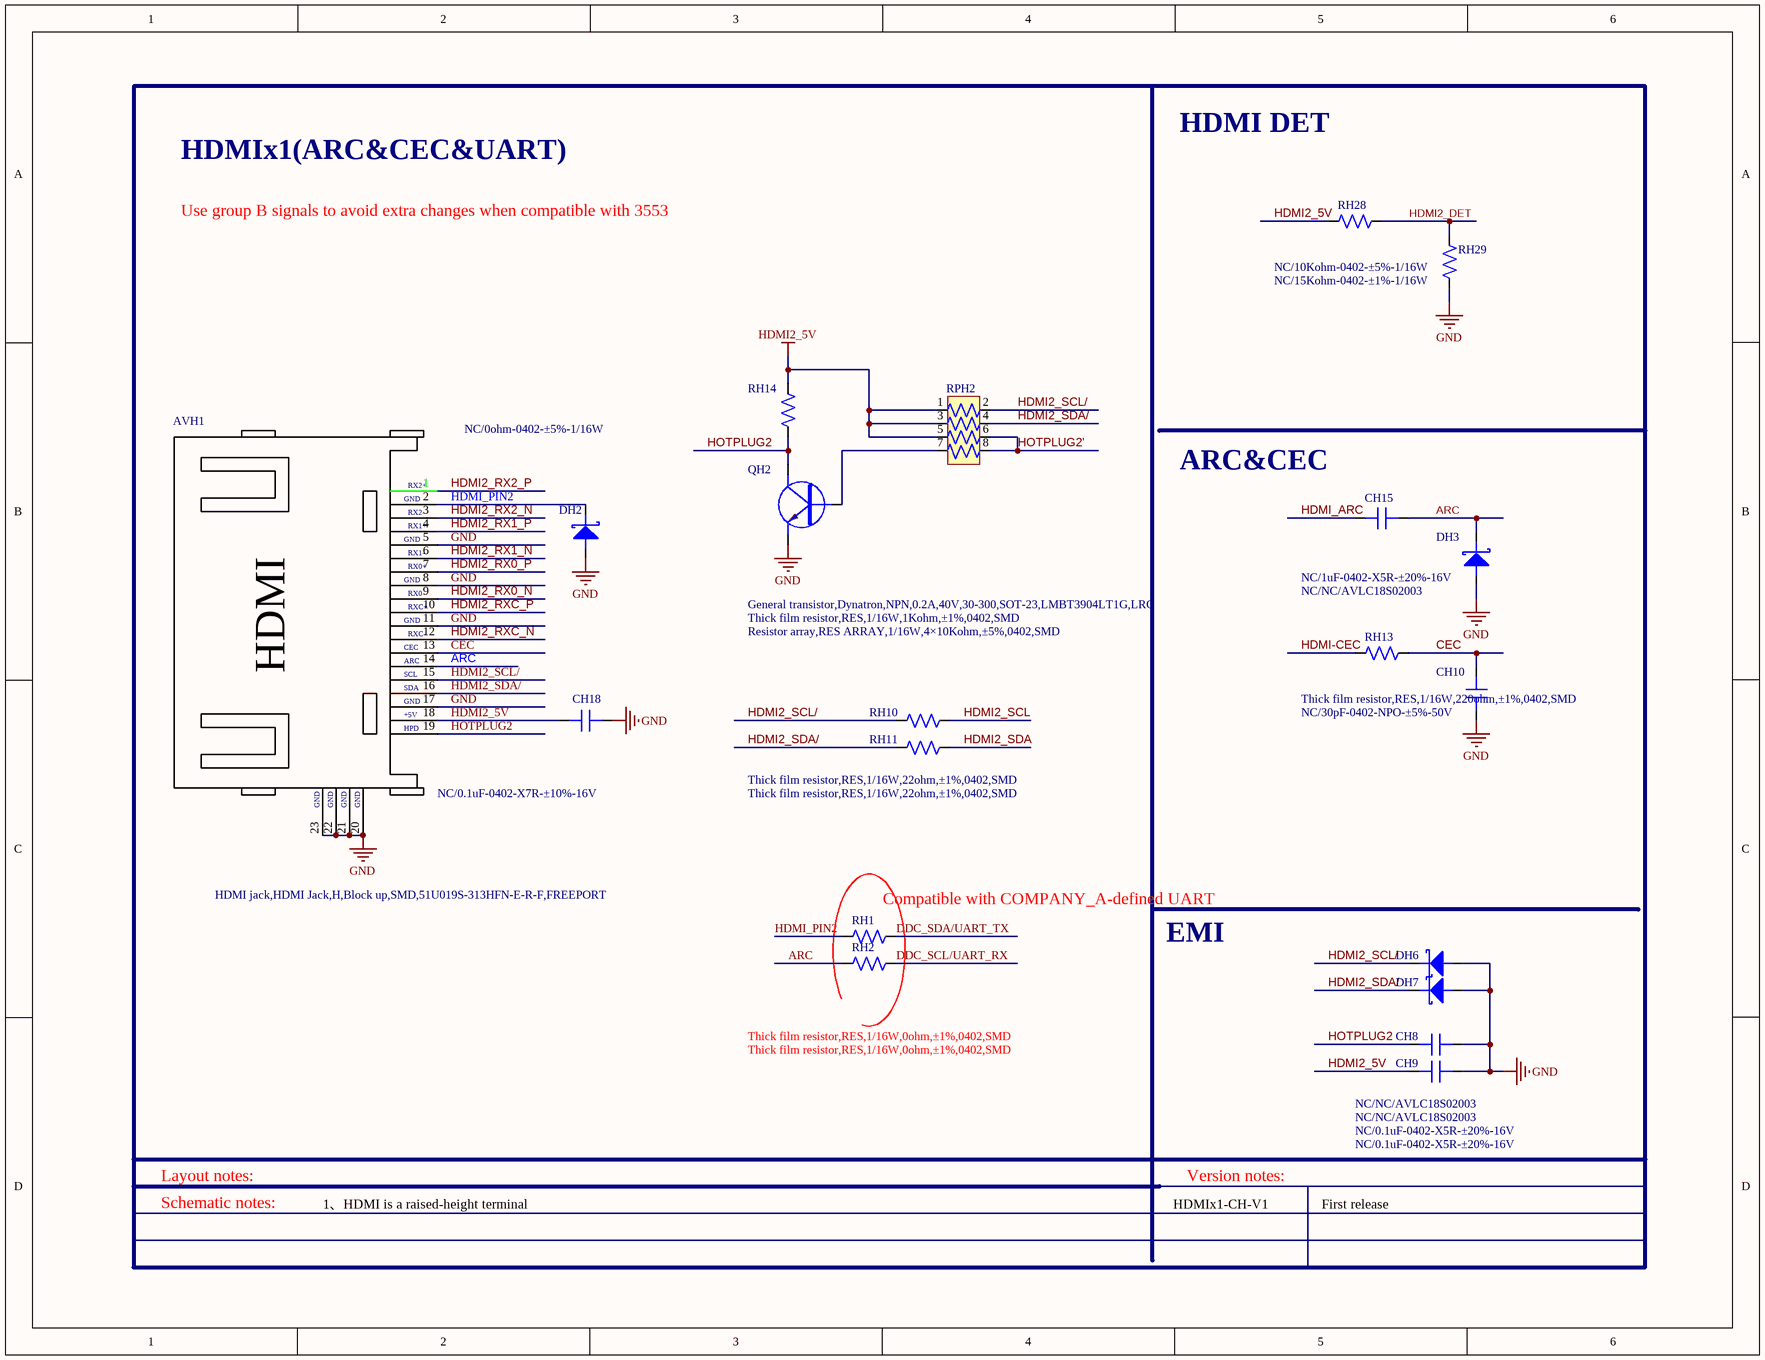
[diagram p0: MISC86383-14.SchDoc]
# Altium project MISC86383-33.PrjPCB (part 4 of 8)

## Sheet MISC86383-14.SchDoc
size 330 x 254 mm

### Parts
AVH1  HDMI jack,HDMI Jack,H,Block up,SMD,51U019S-313HFN-E-R-F,FREEPORT  [HDMI-HS-11]
CH8  NC/0.1uF-0402-X5R-±20%-16V  [C0402]
CH9  NC/0.1uF-0402-X5R-±20%-16V  [C0402]
CH10  NC/30pF-0402-NPO-±5%-50V  [C0402]
CH15  NC/1uF-0402-X5R-±20%-16V  [C0402]
CH18  NC/0.1uF-0402-X7R-±10%-16V  [C0402]
DH2  NC/0ohm-0402-±5%-1/16W  [DIODE-S0402]
DH3  NC/NC/AVLC18S02003  [DIODE-S0402]
DH6  NC/NC/AVLC18S02003  [DIODE-S0402]
DH7  NC/NC/AVLC18S02003  [DIODE-S0402]
QH2  General transistor,Dynatron,NPN,0.2A,40V,30-300,SOT-23,LMBT3904LT1G,LRC  [SOT-23]
RH1  Thick film resistor,RES,1/16W,0ohm,±1%,0402,SMD  [R0402]
RH2  Thick film resistor,RES,1/16W,0ohm,±1%,0402,SMD  [R0402]
RH10  Thick film resistor,RES,1/16W,22ohm,±1%,0402,SMD  [R0402]
RH11  Thick film resistor,RES,1/16W,22ohm,±1%,0402,SMD  [R0402]
RH13  Thick film resistor,RES,1/16W,220ohm,±1%,0402,SMD  [R0402]
RH14  Thick film resistor,RES,1/16W,1Kohm,±1%,0402,SMD  [R0402]
RH28  NC/10Kohm-0402-±5%-1/16W  [R0402]
RH29  NC/15Kohm-0402-±1%-1/16W  [R0402]
RPH2  Resistor array,RES ARRAY,1/16W,4×10Kohm,±5%,0402,SMD  [RA0402]

### Nets
GND: AVH1.5 AVH1.8 AVH1.11 AVH1.17 AVH1.20 AVH1.21 AVH1.22 AVH1.23 CH8.1 CH9.1 CH10.1 CH18.1 DH2.A DH3.A DH6.A DH7.A QH2.E RH29.2
HDMI2_5V: AVH1.18 CH9.2 CH18.2 RH14.2 RH28.2 RPH2.1 RPH2.3 RPH2.5
ARC: AVH1.14 CH15.1 DH3.K RH2.1
CEC: AVH1.13 CH10.2 RH13.1
DDC_SCL/UART_RX: RH2.2
DDC_SDA/UART_TX: RH1.2
HDMI2_DET: RH28.1 RH29.1
HDMI2_RX0_N: AVH1.9
HDMI2_RX0_P: AVH1.7
HDMI2_RX1_N: AVH1.6
HDMI2_RX1_P: AVH1.4
HDMI2_RX2_N: AVH1.3
HDMI2_RX2_P: AVH1.1
HDMI2_RXC_N: AVH1.12
HDMI2_RXC_P: AVH1.10
HDMI2_SCL: RH10.1
HDMI2_SCL/: AVH1.15 DH6.K RH10.2 RPH2.2
HDMI2_SDA: RH11.1
HDMI2_SDA/: AVH1.16 DH7.K RH11.2 RPH2.4
HDMI-CEC: RH13.2
HDMI_ARC: CH15.2
HDMI_PIN2: AVH1.2 DH2.K RH1.1
HOTPLUG2: AVH1.19 CH8.2 QH2.C RH14.1
HOTPLUG2': RPH2.6 RPH2.8
NetQH2_B: QH2.B RPH2.7

### Notes on the sheet
- HDMIx1(ARC&CEC&UART)
- HDMI DET
- Use group B signals to avoid extra changes when compatible with 3553
- ARC&CEC
- (near RH1) Compatible with COMPANY_A-defined UART
- EMI
- Layout notes:
- Schematic notes:
- 1、HDMI is a raised-height terminal
- HDMIx1-CH-V1
- Version notes:
- First release

### Library data of the parts
AVH1 = XXX.XXX.0001809-D: HDMI jack,HDMI Jack,H,Block up,SMD,51U019S-313HFN-E-R-F,FREEPORT-D
CH8 CH9 CH18 = 0.1uF-0402-Y5V-+80%-20%-16V-D
CH10 = 33pF-0402-NPO-±5%-50V-D
CH15 = 1uF-0402-X5R-±20%-16V-D
DH2 DH3 DH6 DH7 = AVLC18S02003-D
QH2 = MMBT3904(f≥350MHz)-D-NPN: Q-NPN-#-#-#
RH1 RH2 = 0ohm-0402-±5%-1/16W-D
RH10 RH11 = 10Kohm-0402-±5%-1/16W-D
RH13 RH28 RH29 = 220ohm-0402-±5%-1/16W-D
RH14 = 1Kohm-0402-±5%-1/16W-D
RPH2 = 4*100ohm-0402-±5%-1/16W-D

## Sheet MISC86383-15.SchDoc
size 330 x 228 mm
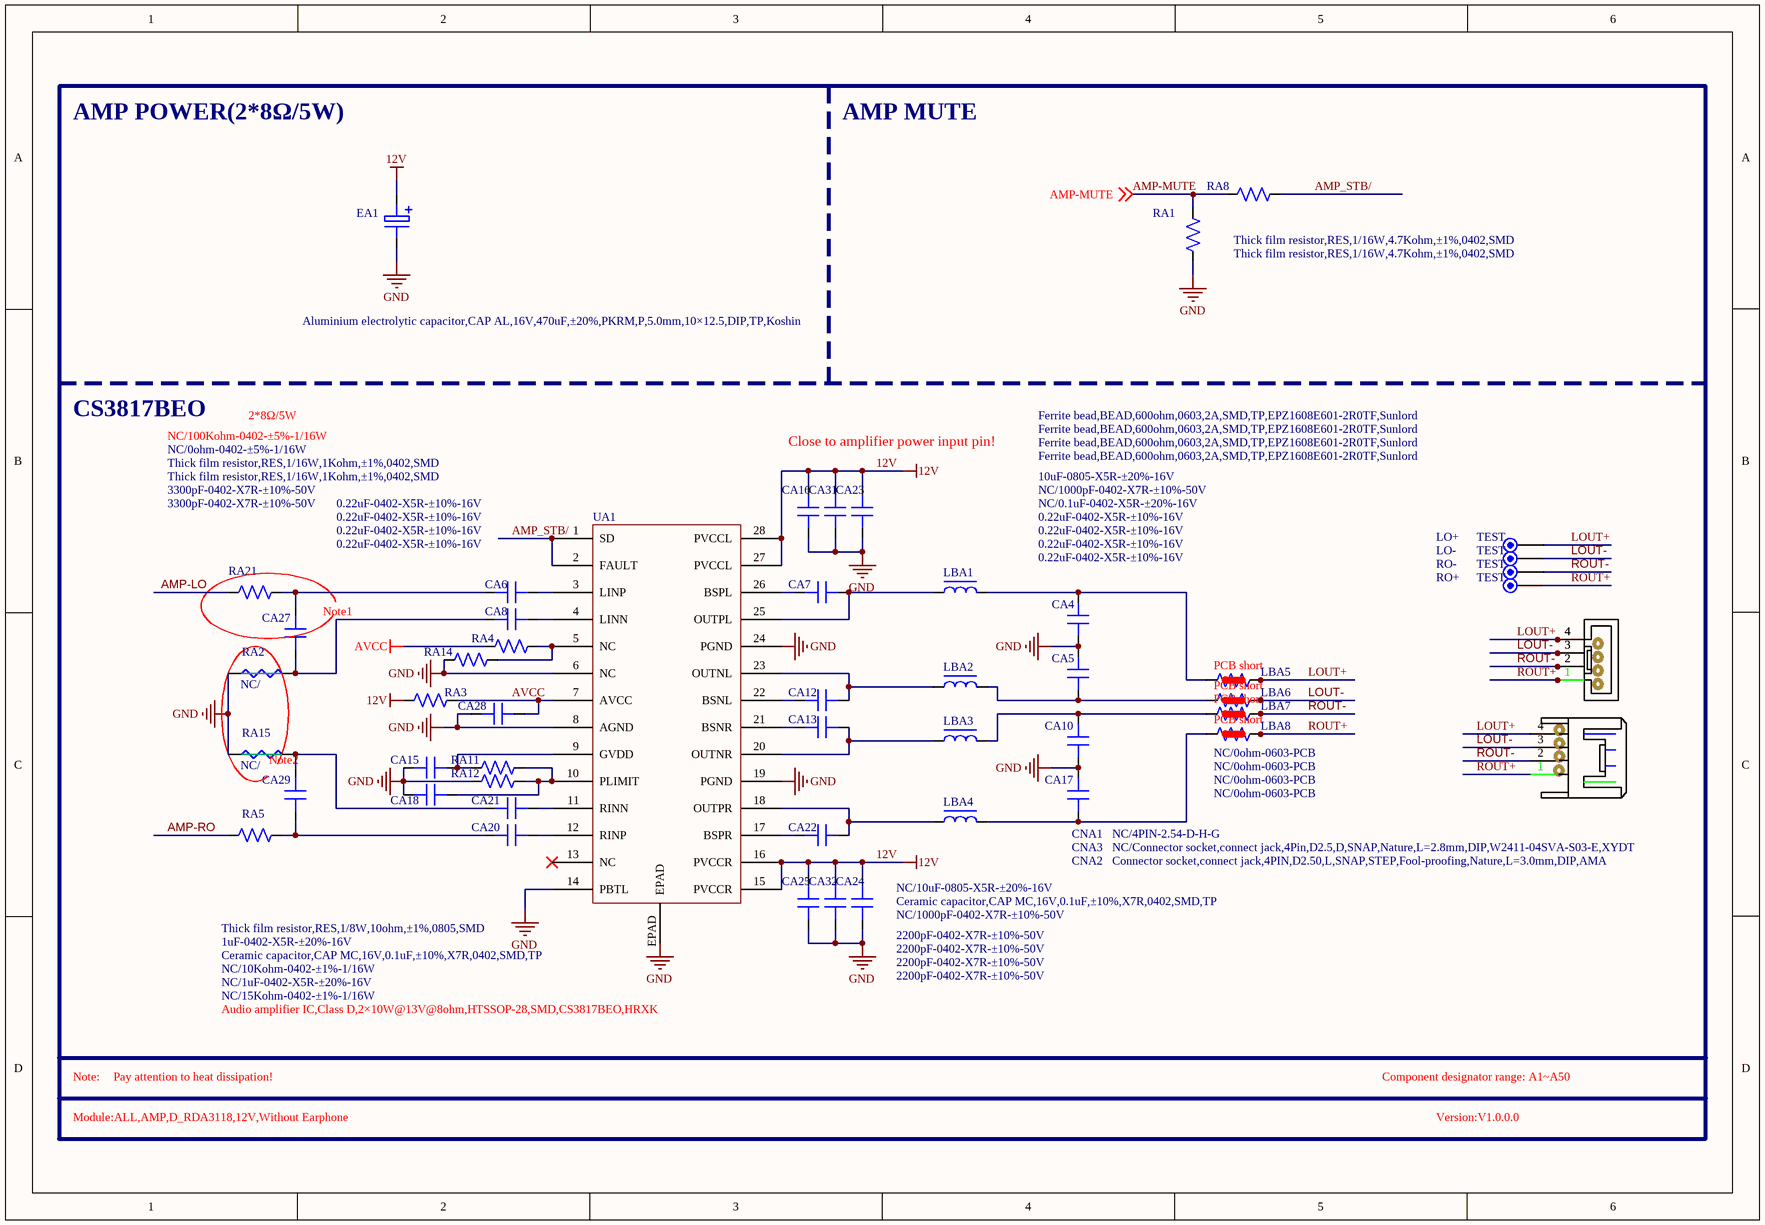
[diagram p1: MISC86383-15.SchDoc]

### Parts
CA4  2200pF-0402-X7R-±10%-50V  [C0402]
CA5  2200pF-0402-X7R-±10%-50V  [C0402]
CA6  0.22uF-0402-X5R-±10%-16V  [C0402]
CA7  0.22uF-0402-X5R-±10%-16V  [C0402]
CA8  0.22uF-0402-X5R-±10%-16V  [C0402]
CA10  2200pF-0402-X7R-±10%-50V  [C0402]
CA12  0.22uF-0402-X5R-±10%-16V  [C0402]
CA13  0.22uF-0402-X5R-±10%-16V  [C0402]
CA15  Ceramic capacitor,CAP MC,16V,0.1uF,±10%,X7R,0402,SMD,TP  [C0402]
CA16  NC/1000pF-0402-X7R-±10%-50V  [C0402]
CA17  2200pF-0402-X7R-±10%-50V  [C0402]
CA18  NC/1uF-0402-X5R-±20%-16V  [C0402]
CA20  0.22uF-0402-X5R-±10%-16V  [C0402]
CA21  0.22uF-0402-X5R-±10%-16V  [C0402]
CA22  0.22uF-0402-X5R-±10%-16V  [C0402]
CA23  NC/0.1uF-0402-X5R-±20%-16V  [C0402]
CA24  Ceramic capacitor,CAP MC,16V,0.1uF,±10%,X7R,0402,SMD,TP  [C0402]
CA25  NC/1000pF-0402-X7R-±10%-50V  [C0402]
CA27  3300pF-0402-X7R-±10%-50V  [C0402]
CA28  1uF-0402-X5R-±20%-16V  [C0402]
CA29  3300pF-0402-X7R-±10%-50V  [C0402]
CA31  10uF-0805-X5R-±20%-16V  [C0805]
CA32  NC/10uF-0805-X5R-±20%-16V  [C0805]
CNA1  NC/4PIN-2.54-D-H-G  [SIP4/2.54D-1]
CNA2  Connector socket,connect jack,4PIN,D2.50,L,SNAP,STEP,Fool-proofing,Nature,L=3.0mm,DIP,AMA  [SIP4H/2.5D-7]
CNA3  NC/Connector socket,connect jack,4Pin,D2.5,D,SNAP,Nature,L=2.8mm,DIP,W2411-04SVA-S03-E,XYDT  [SIP4/2.5D-2]
EA1  Aluminium electrolytic capacitor,CAP AL,16V,470uF,±20%,PKRM,P,5.0mm,10×12.5,DIP,TP,Koshin  [EC(10*12.5)-V-5]
LBA1  Ferrite bead,BEAD,600ohm,0603,2A,SMD,TP,EPZ1608E601-2R0TF,Sunlord  [L0603]
LBA2  Ferrite bead,BEAD,600ohm,0603,2A,SMD,TP,EPZ1608E601-2R0TF,Sunlord  [L0603]
LBA3  Ferrite bead,BEAD,600ohm,0603,2A,SMD,TP,EPZ1608E601-2R0TF,Sunlord  [L0603]
LBA4  Ferrite bead,BEAD,600ohm,0603,2A,SMD,TP,EPZ1608E601-2R0TF,Sunlord  [L0603]
LBA5  NC/0ohm-0603-PCB  [R0603SC]
LBA6  NC/0ohm-0603-PCB  [R0603SC]
LBA7  NC/0ohm-0603-PCB  [R0603SC]
LBA8  NC/0ohm-0603-PCB  [R0603SC]
LO+  TEST  [TP]
LO-  TEST  [TP]
RA1  Thick film resistor,RES,1/16W,4.7Kohm,±1%,0402,SMD  [R0402]
RA2  NC/  [GND]
RA3  Thick film resistor,RES,1/8W,10ohm,±1%,0805,SMD  [R0805]
RA4  NC/100Kohm-0402-±5%-1/16W  [R0402]
RA5  Thick film resistor,RES,1/16W,1Kohm,±1%,0402,SMD  [R0402]
RA8  Thick film resistor,RES,1/16W,4.7Kohm,±1%,0402,SMD  [R0402]
RA11  NC/10Kohm-0402-±1%-1/16W  [R0402]
RA12  NC/15Kohm-0402-±1%-1/16W  [R0402]
RA14  NC/0ohm-0402-±5%-1/16W  [R0402]
RA15  NC/  [GND]
RA21  Thick film resistor,RES,1/16W,1Kohm,±1%,0402,SMD  [R0402]
RO+  TEST  [TP]
RO-  TEST  [TP]
UA1  Audio amplifier IC,Class D,2×10W@13V@8ohm,HTSSOP-28,SMD,CS3817BEO,HRXK  [SSOP28/0.65-5]

### Nets
12V: CA16.2 CA23.2 CA24.2 CA25.2 CA31.2 CA32.2 EA1.1 RA3.1 UA1.15(PVCCR) UA1.16(PVCCR) UA1.27(PVCCL) UA1.28(PVCCL)
AVCC: CA28.2 RA3.2 RA4.2 UA1.7(AVCC)
GND: CA4.2 CA5.2 CA10.2 CA15.2 CA16.1 CA17.1 CA18.2 CA23.1 CA24.1 CA25.1 CA28.1 CA31.1 CA32.1 EA1.2 RA1.1 RA2.JP_2K RA12.2 RA14.1 RA15.JP_2K UA1.6(NC) UA1.8(AGND) UA1.14(PBTL) UA1.19(PGND) UA1.24(PGND) UA1.EPAD
AMP-LO: RA21.1
AMP-MUTE: RA1.2 RA8.1 ; off-sheet AMP-MUTE
AMP-RO: RA5.1
AMP_STB/: RA8.2 UA1.1(SD) UA1.2(FAULT)
LOUT+: CNA1.4 CNA2.4 CNA3.4 LBA5.2 LBA5.3 LO+.1
LOUT-: CNA1.3 CNA2.3 CNA3.3 LBA6.2 LBA6.3 LO-.1
ROUT+: CNA1.1 CNA2.1 CNA3.1 LBA8.2 LBA8.3 RO+.1
ROUT-: CNA1.2 CNA2.2 CNA3.2 LBA7.2 LBA7.3 RO-.1
NetCA4_1: CA4.1 LBA1.2 LBA5.1
NetCA5_1: CA5.1 LBA2.2 LBA6.1
NetCA6_1: CA6.1 UA1.3(LINP)
NetCA6_2: CA6.2 CA27.1 RA21.2
NetCA7_1: CA7.1 UA1.26(BSPL)
NetCA7_2: CA7.2 LBA1.1 UA1.25(OUTPL)
NetCA8_1: CA8.1 UA1.4(LINN)
NetCA8_2: CA8.2 CA27.2 RA2.JP_1K
NetCA10_1: CA10.1 LBA3.2 LBA7.1
NetCA12_1: CA12.1 UA1.22(BSNL)
NetCA12_2: CA12.2 LBA2.1 UA1.23(OUTNL)
NetCA13_1: CA13.1 UA1.21(BSNR)
NetCA13_2: CA13.2 LBA3.1 UA1.20(OUTNR)
NetCA15_1: CA15.1 RA11.2 UA1.9(GVDD)
NetCA17_2: CA17.2 LBA4.2 LBA8.1
NetCA18_1: CA18.1 RA11.1 RA12.1 UA1.10(PLIMIT)
NetCA20_1: CA20.1 UA1.12(RINP)
NetCA20_2: CA20.2 CA29.1 RA5.2
NetCA21_1: CA21.1 UA1.11(RINN)
NetCA21_2: CA21.2 CA29.2 RA15.JP_1K
NetCA22_1: CA22.1 UA1.17(BSPR)
NetCA22_2: CA22.2 LBA4.1 UA1.18(OUTPR)
NetRA4_1: RA4.1 RA14.2 UA1.5(NC)

Not connected (* = marked no-connect by the designer): UA1 13(NC)*

### Notes on the sheet
- AMP POWER(2*8Ω/5W)
- AMP MUTE
- CS3817BEO
- 2*8Ω/5W
- Close to amplifier power input pin!
- (near CA27) Note1
- (near RA15) Note2
- Note:
- Pay attention to heat dissipation!
- Component designator range: A1~A50
- Module:ALL,AMP,D_RDA3118,12V,Without Earphone
- Version:V1.0.0.0

### Library data of the parts
CA4 CA5 CA10 CA16 CA17 CA25 CA27 CA29 = 1000pF-0402-X7R-±10%-50V-D
CA6 CA8 CA20 CA21 = 0.22uF-0402-X5R-±10%-16V-D
CA7 CA12 CA13 CA22 = 0.22uF-0402-Y5V-+80%-20%-16V-D
CA15 CA18 = 1uF-0402-X5R-±20%-16V-D
CA23 CA24 CA28 = 0.1uF-0402-Y5V-+80%-20%-16V-D
CA31 CA32 = 10uF-0603-X5R-±20%-6.3V-D
CNA1 = 4PIN-2.54-D-H-G-DHMI
CNA2 = XXX.XXX.0001836-DLMI: Connector socket,connect jack,4PIN,D2.50,L,SNAP,STEP,Fool-proofing,Nature,L=3.0mm,DIP,AMA-DLMI
CNA3 = 4PIN-2.54-D-H-G-带扣-B-DHMI
EA1 = 470uF-25V-±20%-10×12-105℃-YE-编带-F=5.0(Elite)-DHAI: Electrolytic
LBA1-LBA4 = 004.004.0000104-D: Multilayer inductor,HF Inductor,220nH,±5%,0603,SMD,SWI0603F-R22J,Tai-tech-D
LBA5-LBA8 = 0ohm-0603-PCB-D
RA1 RA8 = 100ohm-0402-±5%-1/16W-D
RA2 RA15 = GND: Manufacturer: Panasonic; Part Number: ERJ3GEYJ473V; Right: 20; Bottom: 30; CLASS: Discrete; Comments: Digikey
RA3 = 10ohm-0805-±5%-1/8W-D
RA4 = 47Kohm-0402-±5%-1/16W-D
RA5 RA21 = 180ohm-0402-±5%-1/16W-D
RA11 = 12Kohm-0402-±5%-1/16W-D
RA12 = 9K1ohm-0402-±5%-1/16W-D
RA14 = 0ohm-0402-±5%-1/16W-D
UA1 = 音频功放,IC Audio AMP,Class D,2×9W@13V@8ohm,HTSSOP28,SMD,TPA3136D2,TI-D

## Sheet MISC86383-16.SchDoc
size 482 x 304 mm
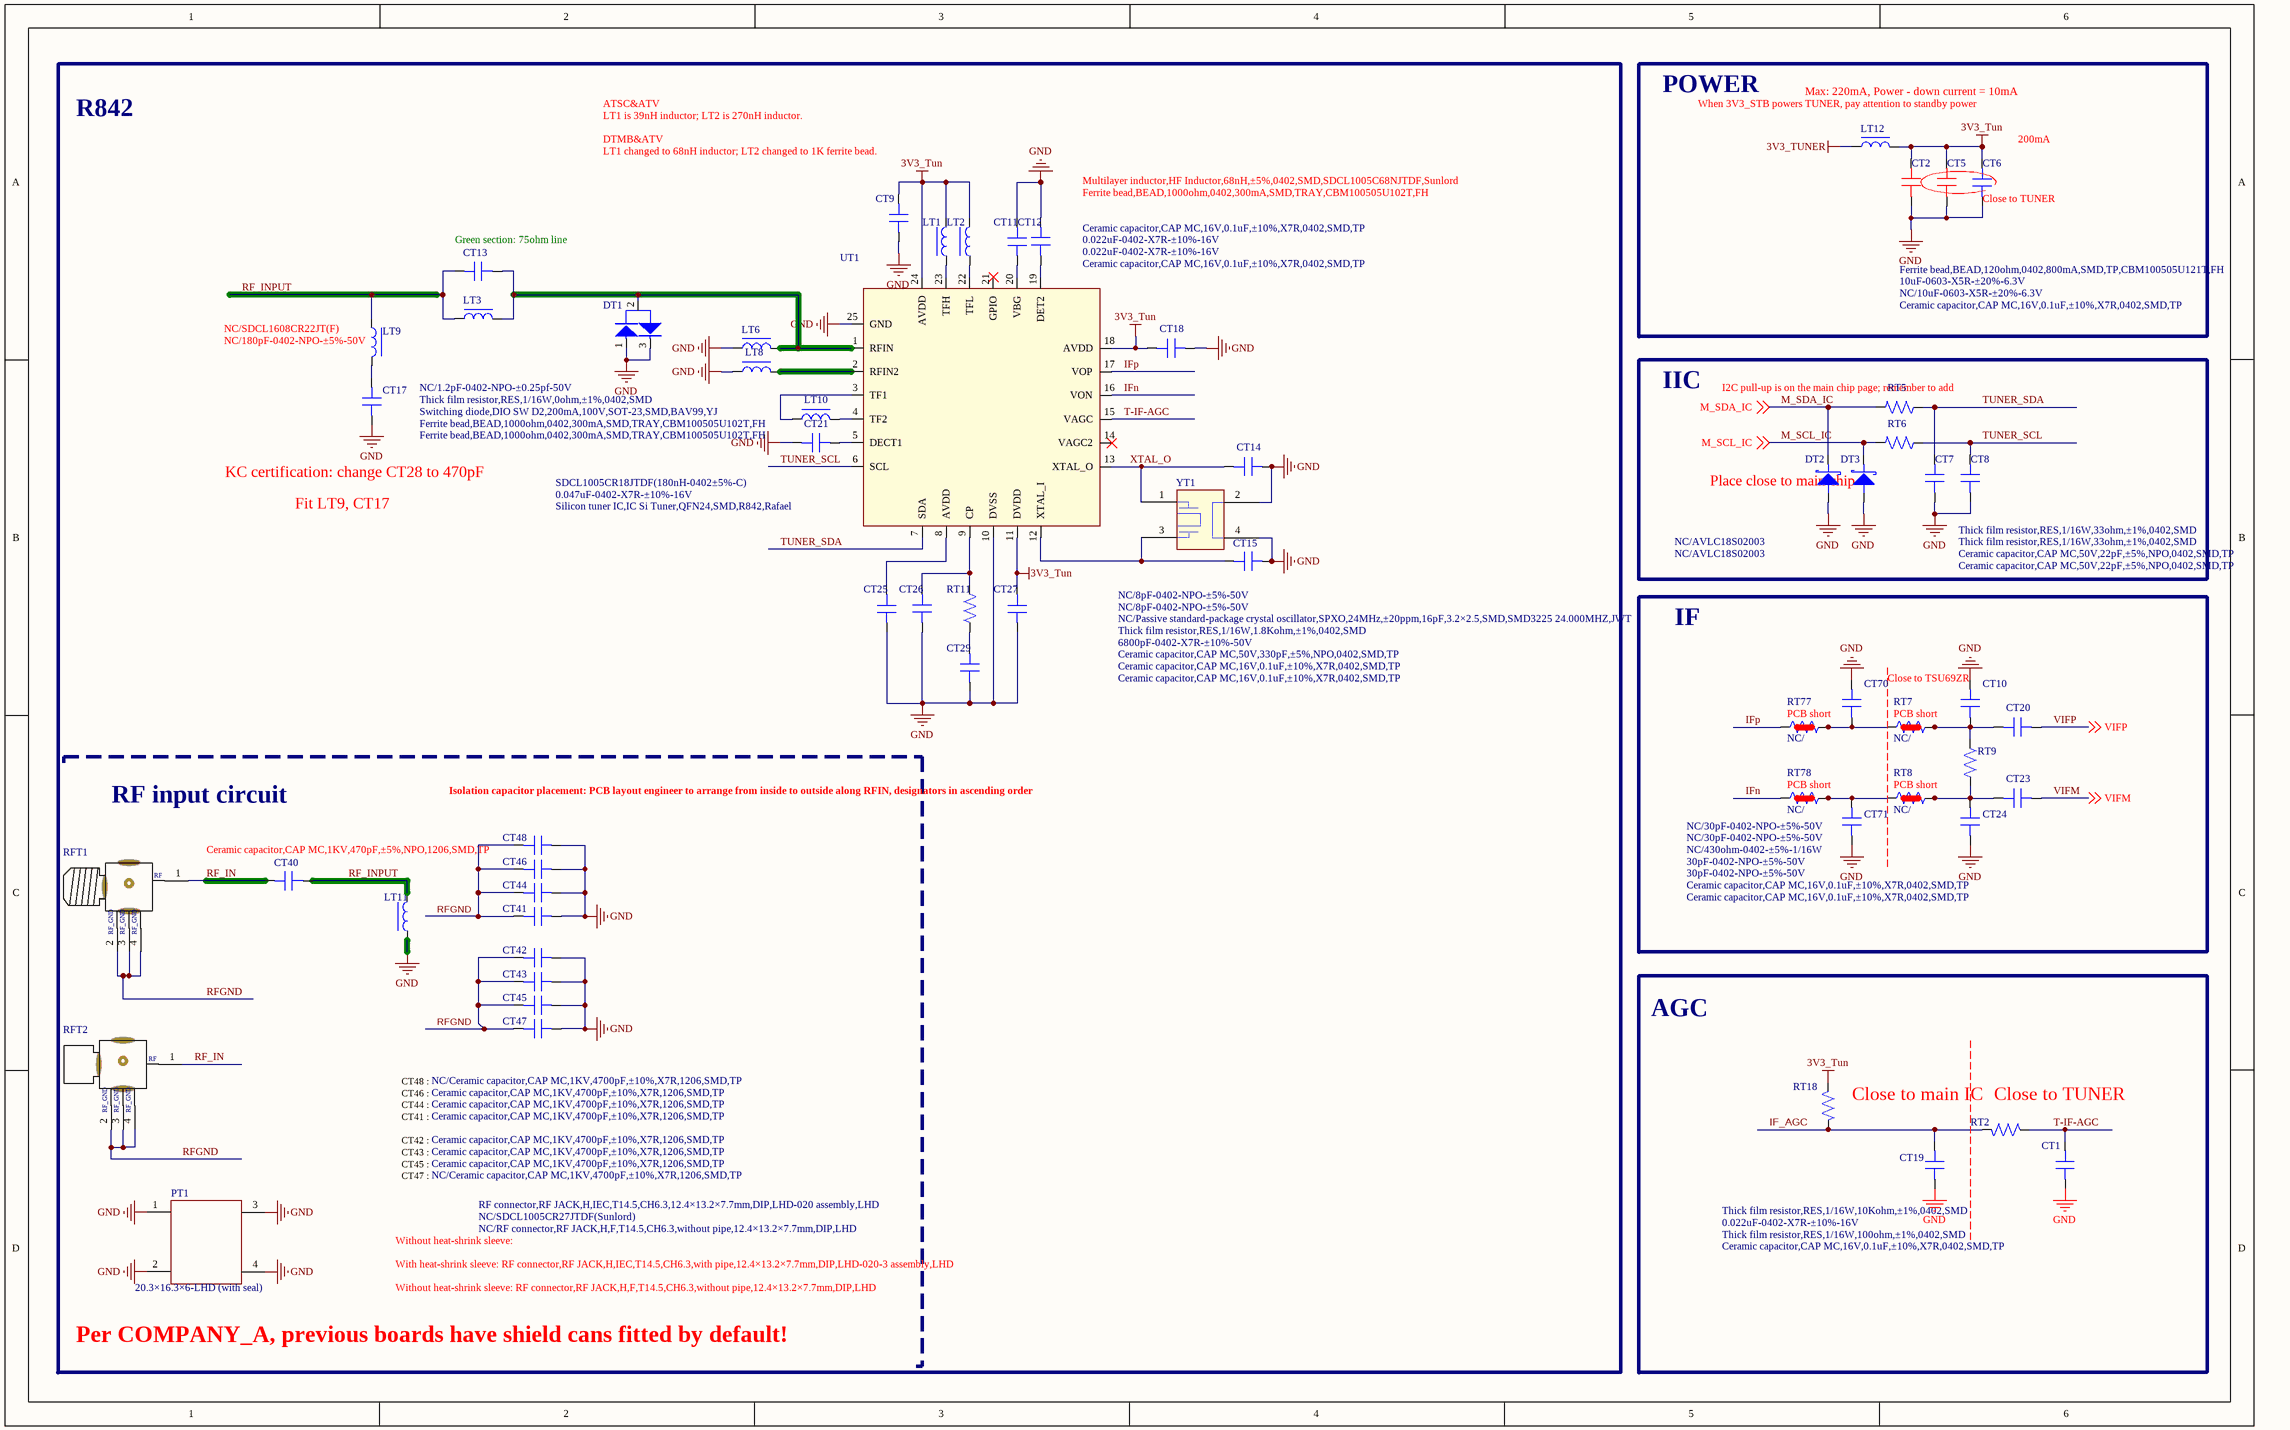
[diagram p2: MISC86383-16.SchDoc]

### Parts
CT1  Ceramic capacitor,CAP MC,16V,0.1uF,±10%,X7R,0402,SMD,TP  [C0402]
CT2  10uF-0603-X5R-±20%-6.3V  [C0603]
CT5  NC/10uF-0603-X5R-±20%-6.3V  [C0603]
CT6  Ceramic capacitor,CAP MC,16V,0.1uF,±10%,X7R,0402,SMD,TP  [C0402]
CT7  Ceramic capacitor,CAP MC,50V,22pF,±5%,NPO,0402,SMD,TP  [C0402]
CT8  Ceramic capacitor,CAP MC,50V,22pF,±5%,NPO,0402,SMD,TP  [C0402]
CT9  Ceramic capacitor,CAP MC,16V,0.1uF,±10%,X7R,0402,SMD,TP  [C0402]
CT10  30pF-0402-NPO-±5%-50V  [C0402]
CT11  0.022uF-0402-X7R-±10%-16V  [C0402]
CT12  0.022uF-0402-X7R-±10%-16V  [C0402]
CT13  NC/1.2pF-0402-NPO-±0.25pf-50V  [C0402]
CT14  NC/8pF-0402-NPO-±5%-50V  [C0402]
CT15  NC/8pF-0402-NPO-±5%-50V  [C0402]
CT17  NC/180pF-0402-NPO-±5%-50V  [C0402]
CT18  Ceramic capacitor,CAP MC,16V,0.1uF,±10%,X7R,0402,SMD,TP  [C0402]
CT19  0.022uF-0402-X7R-±10%-16V  [C0402]
CT20  Ceramic capacitor,CAP MC,16V,0.1uF,±10%,X7R,0402,SMD,TP  [C0402]
CT21  0.047uF-0402-X7R-±10%-16V  [C0402]
CT23  Ceramic capacitor,CAP MC,16V,0.1uF,±10%,X7R,0402,SMD,TP  [C0402]
CT24  30pF-0402-NPO-±5%-50V  [C0402]
CT25  Ceramic capacitor,CAP MC,16V,0.1uF,±10%,X7R,0402,SMD,TP  [C0402]
CT26  Ceramic capacitor,CAP MC,50V,330pF,±5%,NPO,0402,SMD,TP  [C0402]
CT27  Ceramic capacitor,CAP MC,16V,0.1uF,±10%,X7R,0402,SMD,TP  [C0402]
CT29  6800pF-0402-X7R-±10%-50V  [C0402]
CT40  Ceramic capacitor,CAP MC,1KV,470pF,±5%,NPO,1206,SMD,TP  [C1206]
CT41  Ceramic capacitor,CAP MC,1KV,4700pF,±10%,X7R,1206,SMD,TP  [C1206]
CT42  Ceramic capacitor,CAP MC,1KV,4700pF,±10%,X7R,1206,SMD,TP  [C1206]
CT43  Ceramic capacitor,CAP MC,1KV,4700pF,±10%,X7R,1206,SMD,TP  [C1206]
CT44  Ceramic capacitor,CAP MC,1KV,4700pF,±10%,X7R,1206,SMD,TP  [C1206]
CT45  Ceramic capacitor,CAP MC,1KV,4700pF,±10%,X7R,1206,SMD,TP  [C1206]
CT46  Ceramic capacitor,CAP MC,1KV,4700pF,±10%,X7R,1206,SMD,TP  [C1206]
CT47  NC/Ceramic capacitor,CAP MC,1KV,4700pF,±10%,X7R,1206,SMD,TP  [C1206]
CT48  NC/Ceramic capacitor,CAP MC,1KV,4700pF,±10%,X7R,1206,SMD,TP  [C1206]
CT70  NC/30pF-0402-NPO-±5%-50V  [C0402]
CT71  NC/30pF-0402-NPO-±5%-50V  [C0402]
DT1  Switching diode,DIO SW D2,200mA,100V,SOT-23,SMD,BAV99,YJ  [SO-23]
DT2  NC/AVLC18S02003  [DIODE-S0402]
DT3  NC/AVLC18S02003  [DIODE-S0402]
LT1  Multilayer inductor,HF Inductor,68nH,±5%,0402,SMD,SDCL1005C68NJTDF,Sunlord  [L0402]
LT2  Ferrite bead,BEAD,1000ohm,0402,300mA,SMD,TRAY,CBM100505U102T,FH  [L0402]
LT3  Thick film resistor,RES,1/16W,0ohm,±1%,0402,SMD  [L0402]
LT6  Ferrite bead,BEAD,1000ohm,0402,300mA,SMD,TRAY,CBM100505U102T,FH  [L0402]
LT8  Ferrite bead,BEAD,1000ohm,0402,300mA,SMD,TRAY,CBM100505U102T,FH  [L0402]
LT9  NC/SDCL1608CR22JT(F)  [L0603]
LT10  SDCL1005CR18JTDF(180nH-0402±5%-C)  [L0402]
LT11  NC/SDCL1005CR27JTDF(Sunlord)  [L0402]
LT12  Ferrite bead,BEAD,120ohm,0402,800mA,SMD,TP,CBM100505U121T,FH  [L0402]
PT1  20.3×16.3×6-LHD (with seal)  [SHIELD(16*20*6)]
RFT1  NC/RF connector,RF JACK,H,F,T14.5,CH6.3,without pipe,12.4×13.2×7.7mm,DIP,LHD  [T-13.2×12.4×7.7-F14.5]
RFT2  RF connector,RF JACK,H,IEC,T14.5,CH6.3,12.4×13.2×7.7mm,DIP,LHD-020 assembly,LHD  [ANT-IEC14.5-H-4]
RT2  Thick film resistor,RES,1/16W,100ohm,±1%,0402,SMD  [R0402]
RT5  Thick film resistor,RES,1/16W,33ohm,±1%,0402,SMD  [R0402]
RT6  Thick film resistor,RES,1/16W,33ohm,±1%,0402,SMD  [R0402]
RT7  NC/  [R0402SC]
RT8  NC/  [R0402SC]
RT9  NC/430ohm-0402-±5%-1/16W  [R0402]
RT11  Thick film resistor,RES,1/16W,1.8Kohm,±1%,0402,SMD  [R0402]
RT18  Thick film resistor,RES,1/16W,10Kohm,±1%,0402,SMD  [R0402]
RT77  NC/  [R0402SC]
RT78  NC/  [R0402SC]
UT1  Silicon tuner IC,IC Si Tuner,QFN24,SMD,R842,Rafael  [QFN24/0.5-3]
YT1  NC/Passive standard-package crystal oscillator,SPXO,24MHz,±20ppm,16pF,3.2×2.5,SMD,SMD3225 24.000MHZ,JWT  [XTAL-S-10]

### Blocks framed on the sheet
POWER: CT2 CT5 CT6 LT12
IIC: CT7 CT8 DT2 DT3 RT5 RT6
IF: CT10 CT20 CT23 CT24 CT70 CT71 RT7-RT9 RT77 RT78
AGC: CT1 CT19 RT2 RT18

### Nets
3V3_Tun: CT2.2 CT5.2 CT6.1 CT9.1 CT18.2 CT27.1 LT1.1 LT2.2 LT12.2 RT18.1 UT1.11(DVDD) UT1.18(AVDD) UT1.24(AVDD)
3V3_TUNER: LT12.1
GND: CT1.1 CT2.1 CT5.1 CT6.2 CT7.1 CT8.1 CT9.2 CT10.2 CT11.1 CT12.2 CT14.1 CT15.1 CT17.2 CT18.1 CT19.1 CT21.2 CT24.1 CT25.2 CT26.1 CT27.2 CT29.1 CT41.1 CT42.1 CT43.1 CT44.1 CT45.1 CT46.1 CT47.1 CT48.1 CT70.2 CT71.1 DT1.1 DT1.3 DT2.A DT3.A LT6.2 LT8.2 LT11.2 PT1.1 PT1.2 PT1.3 PT1.4 UT1.10(DVSS) UT1.25(GND) YT1.2 YT1.4
IF_AGC: CT19.2 RT2.2 RT18.2
IFn: RT78.1 UT1.16(VON)
IFp: RT77.1 UT1.17(VOP)
M_SCL_IC: DT3.K RT6.2 ; off-sheet M_SCL_IC
M_SDA_IC: DT2.K RT5.2 ; off-sheet M_SDA_IC
RF_IN: CT40.1 RFT1.1 RFT2.1
RF_INPUT: CT13.1 CT40.2 LT3.1 LT9.1 LT11.1
RFGND: CT41.2 CT42.2 CT43.2 CT44.2 CT45.2 CT46.2 CT47.2 CT48.2 RFT1.2 RFT1.3 RFT1.4 RFT2.2 RFT2.3 RFT2.4
T-IF-AGC: CT1.2 RT2.1 UT1.15(VAGC)
TUNER_SCL: CT8.2 RT6.1 UT1.6(SCL)
TUNER_SDA: CT7.2 RT5.1 UT1.7(SDA)
VIFM: CT23.2 ; off-sheet VIFM
VIFP: CT20.2 ; off-sheet VIFP
XTAL_O: CT14.2 UT1.13(XTAL_O) YT1.1
NetCT10_1: CT10.1 CT20.1 RT7.2 RT7.3 RT9.1
NetCT11_2: CT11.2 UT1.20(VBG)
NetCT12_1: CT12.1 UT1.19(DET2)
NetCT13_2: CT13.2 DT1.2 LT3.2 LT6.1 UT1.1(RFIN)
NetCT15_2: CT15.2 UT1.12(XTAL_I) YT1.3
NetCT17_1: CT17.1 LT9.2
NetCT21_1: CT21.1 UT1.5(DECT1)
NetCT23_1: CT23.1 CT24.2 RT8.2 RT8.3 RT9.2
NetCT25_1: CT25.1 UT1.8(AVDD)
NetCT26_2: CT26.2 RT11.2 UT1.9(CP)
NetCT29_2: CT29.2 RT11.1
NetCT70_1: CT70.1 RT7.1 RT77.2 RT77.3
NetCT71_2: CT71.2 RT8.1 RT78.2 RT78.3
NetLT1_2: LT1.2 UT1.23(TFH)
NetLT2_1: LT2.1 UT1.22(TFL)
NetLT8_1: LT8.1 UT1.2(RFIN2)
NetLT10_1: LT10.1 UT1.4(TF2)
NetLT10_2: LT10.2 UT1.3(TF1)

Not connected (* = marked no-connect by the designer): UT1 14(VAGC2)* 21(GPIO)*

### Notes on the sheet
- R842
- ATSC&ATV
- DTMB&ATV
- LT1 is 39nH inductor; LT2 is 270nH inductor.
- When 3V3_STB powers TUNER, pay attention to standby power
- Max: 220mA, Power - down current = 10mA
- (near CT6) 200mA
- (near CT9) LT1 changed to 68nH inductor; LT2 changed to 1K ferrite bead.
- (near CT6) Close to TUNER
- (near CT13) Green section: 75ohm line
- (near RT5) I2C pull-up is on the main chip page; remember to add
- KC certification: change CT28 to 470pF
- Place close to main chip
- Fit LT9, CT17
- (near CT10) Close to TSU69ZR
- Isolation capacitor placement: PCB layout engineer to arrange from inside to outside along RFIN, designators in ascending order
- RF input circuit
- CT46 :
- CT48 :
- CT41 :
- CT42 :
- CT44 :
- Close to main IC
- (near RT2) Close to TUNER
- CT43 :
- CT45 :
- CT47 :
- With heat-shrink sleeve: RF connector,RF JACK,H,IEC,T14.5,CH6.3,with pipe,12.4×13.2×7.7mm,DIP,LHD-020-3 assembly,LHD
- Without heat-shrink sleeve:
- Without heat-shrink sleeve: RF connector,RF JACK,H,F,T14.5,CH6.3,without pipe,12.4×13.2×7.7mm,DIP,LHD
- Per COMPANY_A, previous boards have shield cans fitted by default!

### Library data of the parts
CT1 CT9 CT11 CT18 CT20 CT21 CT23 CT25 CT27 = 0.1uF-0402-Y5V-+80%-20%-16V-D
CT2 CT5 = 004.003.0000383-D: Ceramic capacitor,CAP MC,6.3V,10uF,±20%,X5R,0603,SMD,TP-D
CT6 = 1uF-0402-X5R-±20%-6.3V-D
CT7 CT8 = 004.003.0000530-D: Ceramic capacitor,CAP MC,50V,22pF,±5%,NPO,0402,SMD,TP-D
CT10 CT24 CT70 CT71 = 56pF-0402-NPO-±5%-50V-D
CT12 CT19 = 0.022uF-0402-X7R-±10%-16V-D
CT13 = 1.8pF-0402-NPO-±0.25pF-50V-D
CT14 CT15 = 8pF-0402-NPO-±5%-50V-D
CT17 = 120pF-0402-NPO-±5%-50V-D
CT26 = 330pF-0402-NPO-±5%-50V-D
CT29 = 6800pF-0402-X7R-±10%-50V-D
CT40 = 4700pF-1206-X7R-±10%-1000V-D
CT41-CT48 = 1000pF-1206-X7R-±20%-2000V-D
DT1 = BAV99-BR-D
DT2 DT3 = AVLC18S02003-D
LT1 = SDCL1005C68NJTDF(68nH-0402±5%-C)-D
LT2 LT6 LT8 = 1Kohm-0402-±25%-D
LT3 = 2.2nH-0402-±0.3nH-1/4-D
LT9 = SDCL1005CR33JTDF-D
LT10 = SDCL1608CR22JT(F)-D
LT11 = SDCL1005CR27JTDF(顺络)-D
LT12 = GZ1005U121CTF(120ohm-500mA)-D
PT1 = 20.3×16.3×6-LHD(带封口)-DMI
RFT1 = RF头,RF JACK,H,F,T14.5,CH6.3,without pipe,12.4×13.2×7.7mm,DIP,LHD-DLMI: T-F-6.3mm-#-#
RFT2 = RF头,RF JACK,H,IEC,T14.5,CH6.3,12.4×13.2×7.7mm,DIP,LHD-020组件,LHD-DLMI: T-IEC-6.3mm-#-#
RT2 RT18 = 10Kohm-0402-±5%-1/16W-D
RT5 RT6 = 33ohm-0402-±5%-1/16W-D
RT7 RT8 RT77 RT78 = 0ohm-0402-PCB-D
RT9 = 220ohm-0402-±5%-1/16W-D
RT11 = 1K8ohm-0402-±5%-1/16W-D
UT1 = R840-D
YT1 = 004.009.0000056: Passive standard-package crystal oscillator,SPXO,24MHz,±20ppm,16pF,3.2×2.5,SMD,SMD3225 24.000MHZ,JWT-D